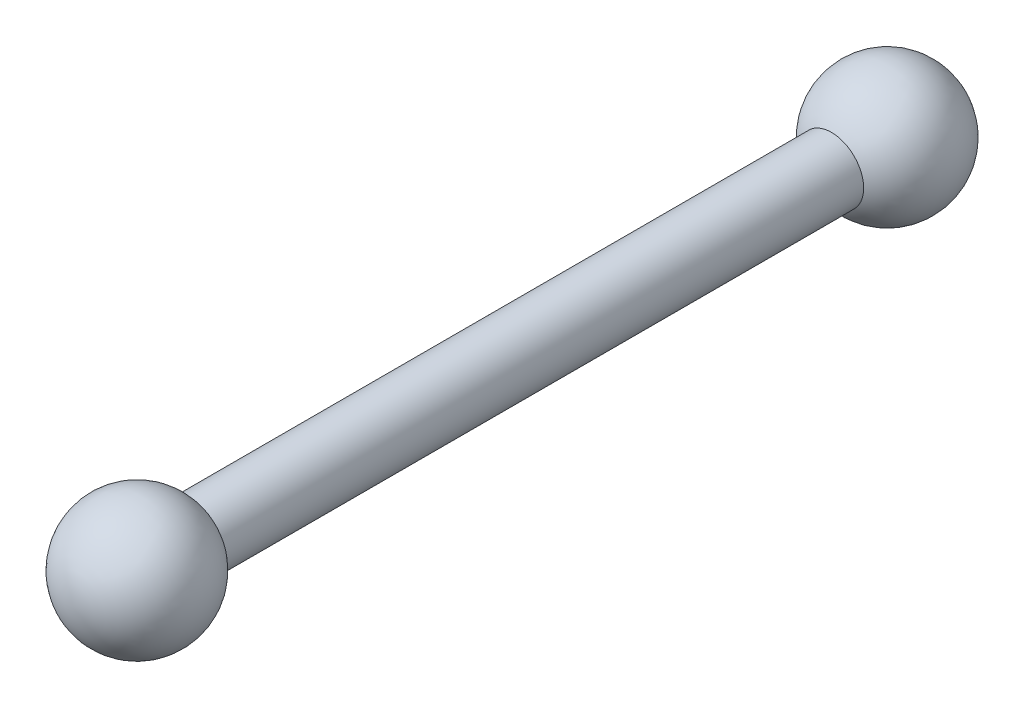
from build123d import *

# Parameters (mm, degrees)
SKETCH1_R           = 15
BOSS_EXTRUDE1_DEPTH = 150


with BuildPart() as part:
    # Sketch1 → Boss-Extrude1 (new, symmetric)
    with BuildSketch(Plane.XY):
        Circle(SKETCH1_R)
    extrude(amount=BOSS_EXTRUDE1_DEPTH, both=True)

    # Sketch2 → Revolve1 (revolve)
    with BuildSketch(Plane(origin=(0, 0, 0), x_dir=(1, 0, 0), z_dir=(0, 1, 0))):
        with BuildLine():
            Line((0, 205), (0, 145))
            ThreePointArc((0, 145), (30, 175), (0, 205))
        make_face()
    revolve1 = revolve(axis=Axis((0, 0, -205), (0, 0, 1)))

    # Mirror1: Revolve1 across plane
    add(revolve1.mirror(Plane.XY))


solid = part.part
